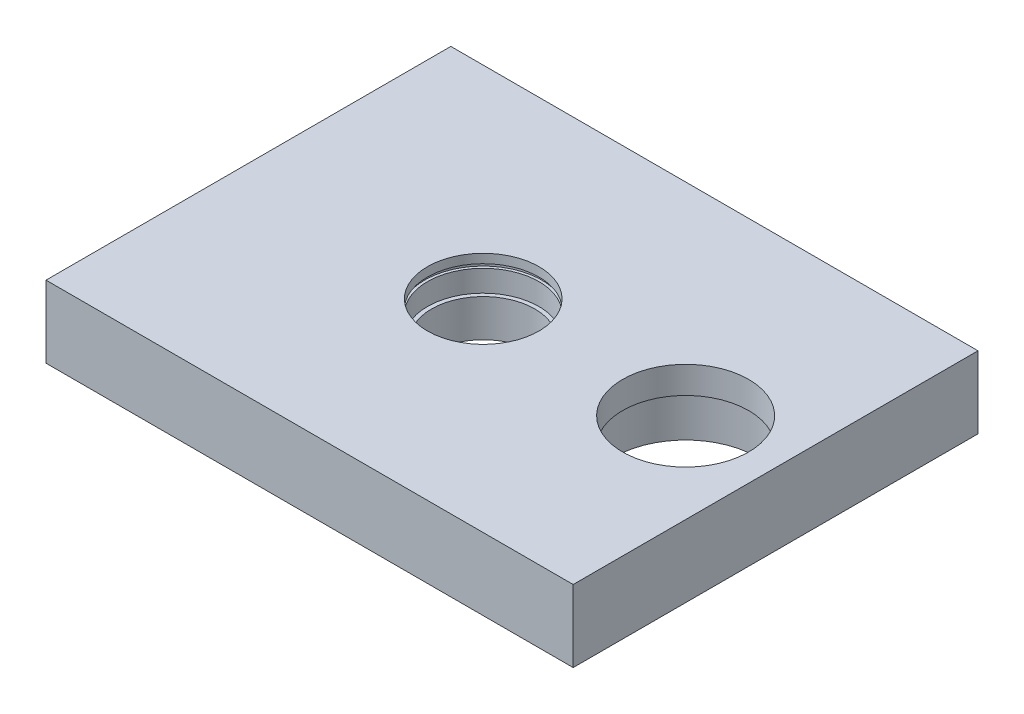
from build123d import *

# Parameters (mm, degrees)
SKETCH_1_W          = 293
SKETCH_1_H          = 225
EXTRUDE_1_DEPTH     = 40
SKETCH_2_R          = 40
CUT_EXTRUDE_1_DEPTH = 25
SKETCH_3_R          = 28.7
CUT_EXTRUDE_2_DEPTH = 189.993386128
SKETCH_4_R          = 35
CUT_EXTRUDE_3_DEPTH = 189.993386128
SKETCH_5_R          = 31
CUT_EXTRUDE_4_DEPTH = 19.2
SKETCH_6_R          = 32.5
CUT_EXTRUDE_5_DEPTH = 2.2


with BuildPart() as part:
    # 草图1 → 凸台-拉伸1 (new body)
    with BuildSketch(Plane(origin=(0, 0, 0), x_dir=(1, 0, 0), z_dir=(0, 1, 0))):
        Rectangle(SKETCH_1_W, SKETCH_1_H)
    extrude(amount=EXTRUDE_1_DEPTH)

    # 草图2 → 切除-拉伸1 (cut)
    with BuildSketch(Plane.XZ):
        with Locations(Location((96.5, 0, 0), (0, 0, 270))):
            Circle(SKETCH_2_R)
    extrude(amount=-CUT_EXTRUDE_1_DEPTH, mode=Mode.SUBTRACT)

    # 草图3 → 切除-拉伸2 (cut, through all)
    with BuildSketch(Plane.XZ):
        with Locations(Location((-16, 0, 0), (0, 0, 270))):
            Circle(SKETCH_3_R)
    extrude(amount=-CUT_EXTRUDE_2_DEPTH, mode=Mode.SUBTRACT)

    # 草图4 → 切除-拉伸3 (cut, through all)
    with BuildSketch(Plane.XZ):
        with Locations(Location((96.5, 0, 0), (0, 0, 270))):
            Circle(SKETCH_4_R)
    extrude(amount=-CUT_EXTRUDE_3_DEPTH, mode=Mode.SUBTRACT)

    # 草图5 → 切除-拉伸4 (cut)
    with BuildSketch(Plane(origin=(0, 40, 0), x_dir=(1, 0, 0), z_dir=(0, 1, 0))):
        with Locations(Location((-16, 0, 0), (0, 0, 270))):
            Circle(SKETCH_5_R)
    extrude(amount=-CUT_EXTRUDE_4_DEPTH, mode=Mode.SUBTRACT)

    # 草图6 → 切除-拉伸5 (cut)
    with BuildSketch(Plane(origin=(0, 35, 0), x_dir=(1, 0, 0), z_dir=(0, 1, 0))):
        with Locations(Location((-16, 0, 0), (0, 0, 270))):
            Circle(SKETCH_6_R)
    extrude(amount=-CUT_EXTRUDE_5_DEPTH, mode=Mode.SUBTRACT)


solid = part.part
